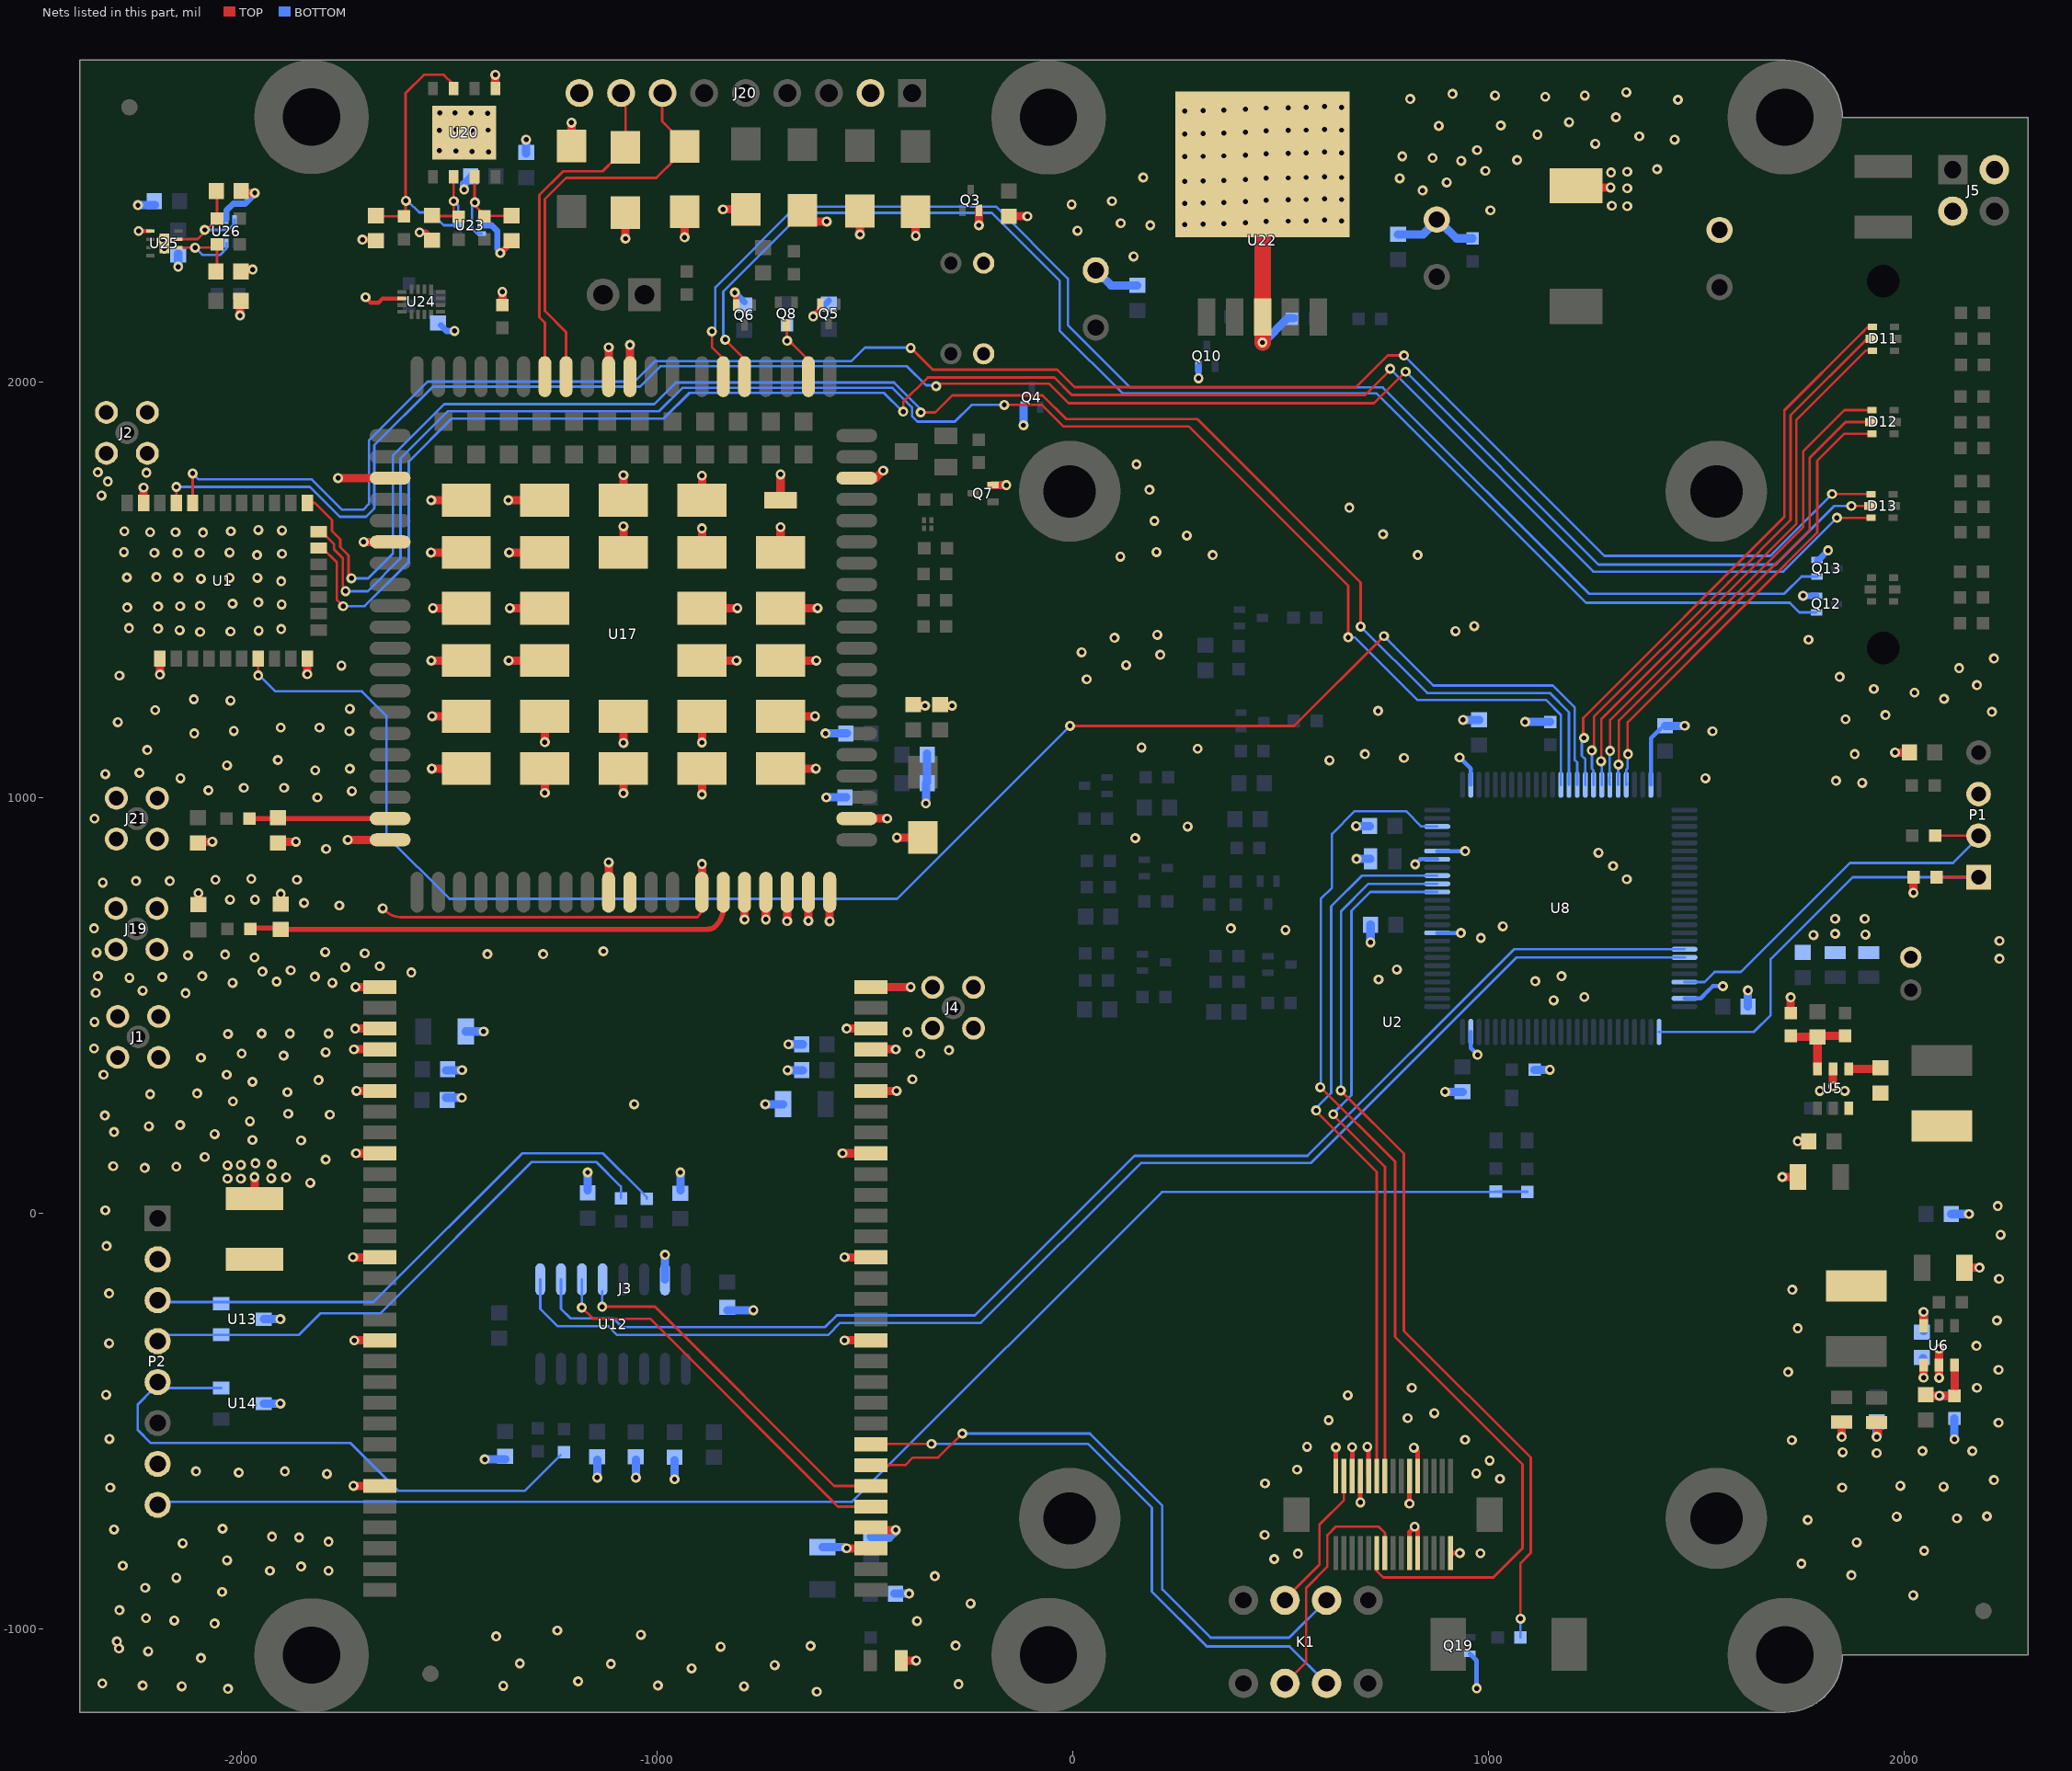
[diagram p0: the nets of this part, all layers, seen from the top]
# Altium PCB MISC84456.PcbDoc (part 3 of 5)
Units mil, origin at the board's own origin, x right, y up, seen from the top; angles counter-clockwise.
Board outline 4685.04 x 3973.82 mil, 4 copper layers (TOP, GND, POWER, BOTTOM), stack 38.4 mil thick; 219 components, 175 nets, 938 pads, 792 vias.

## Via types
v1: diameter 24, hole 12, TOP to BOTTOM, 400 vias
v2: diameter 24, hole 12, TOP to BOTTOM, tented both sides, 388 vias
v3: diameter 40, hole 20, TOP to BOTTOM, 4 vias

## Nets (pads, with @x,y where several pads share a name; then routed paths per layer and width w, separated by ;. In a path a pad name is that pad's centre, name@x,y a point inside that pad or via, vN(x,y) a via of type N, cw(c..) or ccw(c..) an arc to the next point about the centre after c; other vN are vias at no path point) (continued)
232RX-GPS: P2.4 R60.1 U13.1 | length 1332.6
  BOTTOM w6: P2.4@-2194,-293 -2193,-292 -1862,-292 -1810,-240 -1666,-240 -1302,124 -1146,124 -1087,65 R60.1@-1087,36.6
232TX-DB: P2.5 R61.1 U14.2 | length 1381
  BOTTOM w6: P2.5@-2213,-423 -2249,-459 -2249,-520 -2217,-552 -1737,-552 -1622,-667 -1318,-667 R61.1@-1232,-581 ; P2.5@-2201,-413 -2194.4,-419.6 U14.2@-2048.18,-419.6
232TX-GPS: P2.3 R59.1 U13.2 | length 1356.4
  BOTTOM w6: P2.3@-2184,-216 -2181,-213 -1682,-213 -1324,145 -1130,145 -1025,40 R59.1@-1025,35.6
433_CH_SW: R57.2 U8.16 | length 2204.2
  TOP w6: v1(644,296) v1@650.5,289.5 ; v1@647.5,292.5 v1@650.5,289.5 ; v1(1076.5,-974.5) 1076.5,-840.5 1101,-816 1101,-587 796,-282 796,144 v1@650.5,289.5
  BOTTOM w6: v1@645,300 645,727 711.18,793.18 U8.16@876.11,793.18 ; R57.2@1076.5,-1019 v1(1076.5,-974.5)
433_M0: U2.11 U8.17 | length 1875.7
  TOP w6: v1@576,247 578,245 586,245 730.63,100.37 730.63,-129 ; U2.11@730.63,-631.48 730.63,-129 ; 730.63,1.37 730.63,-129
  BOTTOM w6: v1(585,248) 579,248 621,290 ; 621,292 621,739 694.86,812.86 U8.17@876.11,812.86
433_RTK_RX: J3.37 K1.2 | length 1504.3
  TOP w6: J3.37@-485.45,-605 -436,-605 ; -417,-605 -436,-605 ; v1(-266,-529) -324,-587 -385,-587 -403,-605 -436,-605
  BOTTOM w6: v1(-266,-529) 41,-529 215,-703 215,-904 331,-1020 520,-1020 K1.2@610,-930
433_RTK_TX: J3.38 K1.7 | length 1459.9
  TOP w6: J3.38@-455,-554 -430,-554 ; -392,-554 -430,-554 ; v1(-340,-554) -430,-554
  BOTTOM w6: v1(-340,-554) 37,-554 190,-707 190,-909 322,-1041 521,-1041 K1.7@610,-1130
433_RX: K1.3 U2.3 | length 345.8
  TOP w6: K1.3@516,-921 593,-844 593,-748 651.89,-689.11 U2.3@651.89,-631.48
433_SIGNAL: U2.12 U8.23 | length 2654
  TOP w6: v1@594,306 775,125 775,-297 1081,-603 1081,-805 1011,-875 746,-875 730.63,-859.63 U2.12@730.63,-816.52
  BOTTOM w6: v1(595,304) 596,304 596,757 623,784 623,913 678,968 801,968 838.03,930.97 U8.23@876.11,930.97
433_SW: U2.13 U8.15 | length 1657.9
  TOP w6: v1@622.5,240.5 750.31,112.69 U2.13@750.31,-631.48
  BOTTOM w6: v1@624,239 670,285 670,728 715.49,773.49 U8.15@876.11,773.49
  other v1: 626,239
433_TX: K1.6 U2.14 | length 591.9
  TOP w6: K1.6@516,-1124 561,-1079 561,-900 612,-849 612,-773 632,-753 735,-753 750.31,-768.31 U2.14@750.31,-816.52
ACIN: J5.3
ANT_DIV: C103.2 R64.1 U17.35 | length 376.5
  TOP w12.5: R64.1@-1980.5,950 -1944,950 ; -1937,950 -1944,950 ; C103.2@-1903,950 C103.2@-1895,950 ; U17.35@-1679,950.09 U17.35@-1642.02,950.09 ; U17.35@-1656,950 -1944,950
ANT_GNSS: U17.47
ANT_MAIN: C98.2 R62.1 U17.49 | length 1175.6
  TOP w12.5: R62.1@-1978.5,685 -1978.5,687 C98.2@-1901,687 ; C98.2@-1905,683.69 -876.31,683.69 ; -877,684 ccw(c-877,707.9) -860.1,691 ; -859,692 ccw(c-902.84,735.84) U17.49@-840.84,735.84
AP_READY_MODULE: Q8.3 R30.2 U17.2 | length 171.9
  TOP w6: v2(-687.3,2099.3) Q8.3@-687.3,2129.3 ; v2@-682,2099 -664.5,2081.5 -636.12,2053.12 U17.2@-636.12,2013.08
  BOTTOM w6: v2(-687.3,2099.3) R30.2@-687.3,2136.3
BLE_RST: U1.7 U8.40 | length 4123.3
  TOP w6: v1(-1959.35,1294.35) U1.7@-1959.35,1334.99 ; v1(-7,1173) 532,1173 v1(748,1389)
  BOTTOM w6: v1(-1959.35,1294.35) v1@-1954,1294.35 ; v1@-1954,1292 -1918,1256 -1710,1256 -1651,1197 -1651,909 -1499,757 -423,757 v1(-7,1173) ; v1(748,1389) 773.5,1363.5 ; 770,1367 773.5,1363.5 ; U8.40@1212.72,1031.36 1212.72,1085.28 1207,1091 1207,1217 1154,1270 867,1270 773.5,1363.5
BLE_SLP: U1.17 U8.38 | length 4041.4
  TOP w6: U1.17@-1813.69,1640.11 -1806.86,1640.11 -1777,1610.25 -1777,1598 -1756,1577 v1@-1756,1504 ; v1@-165,1944 v1@-163,1946 ; v1@-162,1945 -74,1945 -22,1893 279,1893 662,1510 v1(662,1386)
  BOTTOM w6: v1(-1749,1497) -1696,1497 -1617,1576 -1617,1816 -1503,1930 -995,1930 -939,1986 -434,1986 -387,1939 -387,1918.3 -373.7,1905 -284,1905 -244,1945 v1(-165,1945) ; v1(662,1386) 678,1386 829,1235 1138.23,1235 1173.35,1199.87 U8.38@1173.35,1031.36
BLE_SW: U1.18 U8.39 | length 4087
  TOP w6: U1.18@-1841.24,1709.01 -1823.01,1709.01 -1782,1668 -1782,1642 -1762,1622 -1762,1603 -1742,1583 v1@-1742,1535 ; v1@-362,1927 -331,1927 -290,1968 -73,1968 -16,1911 299,1911 692,1518 v1(692,1412)
  BOTTOM w6: v1(-1735,1528) -1695,1528 -1635,1588 -1635,1824 -1512,1947 -1007,1947 -955,1999 -430,1999 -366,1935 v1(-366,1927) ; v1(692,1412) 852,1252 1147,1252 1193.04,1205.96 U8.39@1193.04,1031.36
BOOT0: P2.8 R37.2 R38.1 | length 3595.1
  BOTTOM w6: P2.8@-2196,-694 -2195,-693 -531,-693 214,52 1015.5,52 R38.1@1017,53.5 ; R38.1@1020.5,52.5 R37.2@1093,52.5
CPU-URX0: U8.69 U12.9 | length 3286.8
  BOTTOM w6: -1281,-219 U12.9@-1281,-158.2 -1281,-229 -1239,-271 -1117,-271 -1096,-292 -589,-292 -560,-263 -221,-263 164,122 573,122 1067,616 U8.69@1472,616
CPU-UTX0: U8.68 U12.10 | length 3167
  BOTTOM w6: U12.10@-1231,-158.2 -1231,-229 -1208,-252 -1105,-252 -1084,-273 -596,-273 -568,-245 -236,-245 148,139 564,139 1060.69,635.69 U8.68@1470.59,635.69
DBG_RXD: D18.2 J20.7 U17.11 | length 898.7
  TOP w6: U17.11@-1219,2038 -1219,2120 -1269.98,2170.98 -1269.98,2440.02 -1219,2491 -1001,2491 -1001,2492 D18.2@-955,2538 ; J20.7@-988,2670 -988,2627 D18.2@-934,2573
DBG_TXD: D19.2 J20.8 U17.12 | length 773.6
  TOP w6: U17.12@-1269.98,2013.08 -1269.98,2142.98 -1283,2156 -1283,2450 -1226,2507 -1131,2507 D19.2@-1101,2537 ; D19.2@-1076,2564.74 J20.8@-1076,2678
DBG_TXD_FC20: J20.9
GND: C1.1 C2.2 C3.2 C4.2 C5.1 C6.2 C7.2 C8.1 C9.1 C10.1 C11.2 C20.1 C21.1 C22.1 C24.2 C26.2 C27.2 C28.2 C29.2 C30.1 C31.1 C32.2 C34.2 C35.2 C36.2 C37.2 C38.1 C40.2 C41.2 C42.2 C43.2 C44.1 C45.2 C46.1 C47.2 C48.2 C49.2 C50.2 C51.2 C52.2 C53.2 C54.2 C55.1 C56.2 C70.2 C71.2 C72.2 C73.2 C74.2 C75.2 C76.2 C77.2 C88.2 C91.2 C92.2 C94.1 C95.1 C96.2 C97.1 C98.1 C99.2 C100.2 C101.2 C102.1 C103.1 C104.2 C105.2 D3.1 D7.2 D8.1 D14.1 D15.1 D16.1 D17.1 D18.1 D19.1 D24.1 J1.2 J1.3 J1.4 J1.5 J2.2 J2.3 J2.4 J2.5 J3.1 J3.3 J3.4 J3.6 J3.9 J3.14 J3.18 J3.25 J3.33 J3.34 J3.43 J3.47 J3.52 J3.55 J3.57 J3.58 J3.60 J4.2 J4.3 J4.4 J4.5 J5.2 J19.2 J19.3 J19.4 J19.5 J20.2 J21.2 J21.3 J21.4 J21.5 L2.2 P1.3 P2.7 Q3.2 Q4.2 Q5.2 Q6.2 Q7.2 Q10.2 Q12.2 Q13.2 Q19.1 R4.1 R7.2 R13.1 R20.1 R36.1 R42.1 R67.1 R68.1 U1.1 U1.10 U1.28 U2.1 U2.5 U2.7 U2.9 U2.19 U2.20 U2.21 U2.22 U2.30 U5.2 U6.2 U8.10 U8.19 U8.20 U8.27 U8.49 U8.74 U8.99 U12.15 U13.3 U14.3 U17.8 U17.9 U17.19 U17.22 U17.36 U17.46 U17.48 U17.50 U17.51 U17.52 U17.53 U17.54 U17.56 U17.72 U17.85 U17.86 U17.87 U17.88 U17.89 U17.90 U17.91 U17.92 U17.93 U17.94 U17.95 U17.96 U17.97 U17.98 U17.99 U17.100 U17.101 U17.102 U17.103 U17.104 U17.105 U17.106 U17.107 U17.108 U17.109 U17.110 U17.111 U17.112 U20.1 U20.9 U22.3 U22.6 U23.2 U24.6 U25.1 U25.9 U26.2 | length 11053.5
  TOP w6: v1@-1654,729 ccw(c-1615.37,767.63) -1615.37,713 -903,713 ccw(c-929.5,739.5) -892.02,739.5 U17.48@-892.02,772.92
  TOP w10: v2(-2246.92,2363.08) U25.1@-2218.15,2363.08 ; v2(-1701,2204) -1688,2191 -1670,2191 -1660.13,2200.87 U24.6@-1613.41,2200.87
  TOP w11: U2.5@671.57,-631.48 v1(671.57,-561.57) ; v1(691.26,-694.74) U2.7@691.26,-631.48 ; v1(708,-561) 710.94,-563.94 U2.9@710.94,-631.48 ; U2.20@809.37,-816.52 809.37,-765.63 v1@817,-758 ; v1(809.37,-697.63) U2.19@809.37,-631.48 ; v1(820,-563) 829.06,-572.06 U2.21@829.06,-631.48 ; v1(822,-753) 829.06,-760.06 U2.22@829.06,-816.52 ; U2.30@907.8,-816.52 v1(930.52,-816.52)
  TOP w12: U2.1@632.2,-631.48 v1(632.2,-562.2)
  TOP w15: v2(-1708.5,2342.5) C37.2@-1676,2342.5 ; v2(-1571,2360) -1557.5,2360 C36.2@-1541,2343.5 ; v2(-1377,2310) -1356,2331 C35.2@-1356,2343.5 ; v2(-813,2215.5) -810.12,2212.62 Q6.2@-810.12,2184.87 ; v2(-624.5,2158) -608,2174.5 Q5.2@-608,2181
  TOP w20: U1.28@-2234.94,1709.01 v1(-2234.94,1746.06) ; v1(-2195.57,1296.43) U1.1@-2195.57,1334.99 ; C102.1@-2104,894.5 v2(-2069.5,894.5) ; C97.1@-2103,740.5 v2(-2103,771) ; C51.2@-2003.18,2270.56 v2(-1972.44,2270.56) ; C50.2@-2003.18,2454.56 v2(-1967.56,2454.56) ; v2(-2003,2160) C52.2@-2003,2201 ; L2.2@-1968,36.97 v2(-1968,88) ; C103.1@-1912,894.5 v2(-1868.5,894.5) ; C98.1@-1905,741.5 v2(-1905,769) ; v1(-1841.24,1297.24) U1.10@-1841.24,1334.99 ; v2(-1767.02,1768.98) U17.19@-1642.02,1768.98 ; v2(-1744.09,898.91) U17.36@-1642.02,898.91 ; v2(-1731,-105) J3.14@-1666.55,-105 ; v1(-1730,-655) J3.25@-1666.55,-655 ; v2(-1729,395) J3.4@-1666.55,395 ; v2(-1728,-305) J3.18@-1666.55,-305 ; v2(-1726,445) J3.3@-1666.55,445 ; v2(-1725,545) J3.1@-1666.55,545 ; v2(-1724,145) J3.9@-1666.55,145 ; v2(-1723,295) J3.6@-1666.55,295 ; v2(-1705.56,1615.44) U17.22@-1631.02,1615.44 ; v2(-1543.85,1589.85) U17.107@-1458.95,1589.85 ; v2(-1543.17,1715.83) U17.112@-1458.95,1715.83 ; v2(-1542.99,1330.01) U17.98@-1458.95,1330.01 ; v2(-1541.83,1070.17) U17.89@-1458.95,1070.17 ; v2(-1540.85,1196.15) U17.94@-1458.95,1196.15 ; v2(-1538.99,1455.99) U17.102@-1458.95,1455.99 ; U20.1@-1389,2706.3 v2(-1389,2739) ; R42.1@-1372,2185.5 v2(-1372,2217) ; v2(-1357.83,1715.83) U17.111@-1269.98,1715.83 ; v2(-1357.01,1330.01) U17.97@-1269.98,1330.01 ; v2(-1355.85,1589.85) U17.106@-1269.98,1589.85 ; v2(-1353.99,1455.99) U17.101@-1269.98,1455.99 ; v2(-1269.98,1012.02) U17.88@-1269.98,1070.17 ; v2(-1269.98,1133.98) U17.93@-1269.98,1196.15 ; D24.1@-1206,2567.74 v2(-1206,2624) ; U17.46@-1116.43,772.92 v2(-1116.43,844.57) ; U17.9@-1116.43,2013.08 v2@-1116.43,2081.43 ; v2(-1081,1011) U17.87@-1081,1070.17 ; v2(-1081,1132) U17.92@-1081,1196.15 ; U17.105@-1081,1589.85 v2(-1081,1653) ; U17.110@-1081,1715.83 v2(-1081,1776) ; v2(-1076,2345) D19.1@-1076,2407.26 ; U17.8@-1065.25,2013.08 v2(-1065.25,2089.25) ; v2(-934,2348) D18.1@-934,2409.26 ; U17.48@-892.02,772.92 v2(-892.02,840.98) ; v2(-892.02,1008.02) U17.86@-892.02,1070.17 ; v2(-892.02,1132.98) U17.91@-892.02,1196.15 ; U17.96@-892.02,1330.01 v2(-809.01,1330.01) ; U17.100@-892.02,1455.99 v2(-807.01,1455.99) ; U17.104@-892.02,1589.85 v2(-892.02,1647.98) ; U17.109@-892.02,1715.83 v2(-892.02,1774.98) ; v2(-841.74,2415.26) D14.1@-787,2415.26 ; v2(-789.66,707.34) U17.50@-789.66,772.92 ; v2(-738.48,707.48) U17.51@-738.48,772.92 ; U17.85@-703.05,1070.17 v2(-618.17,1070.17) ; U17.90@-703.05,1196.15 v2(-620.15,1196.15) ; U17.95@-703.05,1330.01 v2(-617.01,1330.01) ; U17.99@-703.05,1455.99 v2(-614.01,1455.99) ; U17.103@-703.05,1589.85 v2(-703.05,1651.05) ; U17.108@-703.05,1715.83 v2(-703.05,1777.95) ; v2(-687.3,703.3) U17.52@-687.3,772.92 ; D15.1@-651,2413.26 -651,2396 -641,2386 v2(-592,2386) ; v2(-636.12,704.12) U17.53@-636.12,772.92 ; v2(-584.94,703.06) U17.54@-584.94,772.92 ; v2(-554,145) J3.52@-485.45,145 ; v2(-549,-305) J3.43@-485.45,-305 ; v2(-549,-105) J3.47@-485.45,-105 ; v2(-544,-805) J3.33@-485.45,-805 ; v2(-544,445) J3.58@-485.45,445 ; U17.56@-519.98,950.09 v2(-446.91,950.09) ; U17.72@-519.98,1768.98 -474.02,1768.98 v2(-456,1787) ; v2(-512,2355) D16.1@-512,2411.26 ; J3.34@-485.45,-755 -479.45,-761 v2(-426,-761) ; J3.55@-485.45,295 v2(-424,295) ; J3.57@-485.45,395 v2(-426,395) ; J3.60@-485.45,545 v2(-390,545) ; v2(-423.26,904.26) D8.1@-361,904.26 ; D7.2@-412.6,-1075 v2(-377,-1075) ; C73.2@-384,1221.5 v2(-355.5,1221.5) ; v2(-378,2352) D17.1@-378,2409.26 ; C74.2@-319,1221.5 v2(-290.5,1221.5) ; v1(-226,2377) Q3.2@-226,2413.38 ; Q7.2@-192.38,1752 v1(-160,1752) ; C32.2@-154,2398.69 v1(-109.68,2398.69) ; D3.1@1231.13,2468 v2(1293,2468) ; v2(1706,88) C30.1@1743.84,88 ; R13.1@1726,482.5 v2(1726,520) ; v2(1743,174) C31.1@1772.5,174 ; v2(1828,306) U5.2@1828,347.89 ; v2(1849,-537) C42.2@1849,-501.53 ; v2(1933,-537) 1936,-534 C40.2@1936,-508 ; v1(1977,1109) C1.1@2011.69,1109 ; v1(2021.5,771.5) R7.2@2021.5,809 ; v2(2083,-395) U6.2@2083,-364.24 v2(2083,-325) ; C44.1@2144.16,-130 v2(2180,-130)
  TOP w40: v2(456,2095) U22.3@456,2156.23 U22.6@456,2349
  BOTTOM w10: v2(-1701,2204) v2@-1701,2205 ; v1(823,840) 835.23,852.23 U8.19@876.11,852.23 ; U8.10@876.11,675.06 v1(932.94,675.06) ; U8.20@876.11,871.92 v1(943.08,871.92) ; v1(930,1097) 929,1098 956.81,1070.19 U8.27@956.81,1031.36 ; U8.99@956.81,436.88 956.81,398.19 v1(973,382) ; U8.49@1389.89,1031.36 1389.89,1143.89 C3.2@1412,1166 ; U8.74@1470.59,517.58 1509.58,517.58 1527,535 1539,547 v1(1563,547)
  BOTTOM w11: Q19.1@954.56,-1058.68 971,-1075.13 v1(971,-1142)
  BOTTOM w15: U26.2@-2035.68,2391 -2035.68,2412.32 -2019,2429 -1991,2429 v2@-1970,2450 ; C38.1@-1519.5,2136.5 -1506,2123 v2(-1487,2123) ; U23.2@-1421.56,2377 -1398,2377 -1384,2363 -1384,2320 v2@-1377,2313 ; v2(-813,2215.5) C48.2@-790,2192.5 ; v2(-624.5,2158) C47.2@-587,2195.5 ; v1(302,2009) Q10.2@302,2038.38 ; v1(1756,1486) Q12.2@1788.38,1486 ; Q13.2@1789.38,1572 1793,1572 v1(1816,1595)
  BOTTOM w20: v2(-2248.44,2425.56) C45.2@-2207.18,2425.56 ; v2(-2151.68,2277.32) C49.2@-2151.68,2308.06 ; U14.3@-1945.82,-457 v1(-1906,-457) ; U13.3@-1945.82,-254 v1(-1906,-254) ; C8.1@-1507.62,278.76 v2(-1469.75,278.76) ; C9.1@-1507.5,345 v2(-1469,345) ; v2(-1464,2463) -1464,2476.5 C34.2@-1445.5,2495 ; C10.1@-1459.84,438 v2(-1417,438) ; v2(-1414.3,-591.3) C99.2@-1365,-591.3 ; C24.2@-1315,2549.5 v2(-1315,2583) ; C95.1@-1167,56.5 v2(-1167,99) ; v2(-1144,-635) C100.2@-1144,-592.3 ; v2(-1051,-635) C96.2@-1051,-592.4 ; U12.15@-981,-158.2 v2(-981,-99) ; v2(-958,-639) C92.2@-958,-593.4 ; C94.1@-944,55.5 v2(-944,99) ; C88.2@-831,-232.4 v2(-768.4,-232.4) ; v2(-740,263) C5.1@-697.16,263 ; v2(-686.24,344.76) C6.2@-649.62,344.76 ; v2(-684,407) C7.2@-649.5,407 ; C22.1@-602,-801.84 -551.16,-801.84 v2@-548,-805 ; v2(-595,1155) C72.2@-543.5,1155 ; v2(-593,1001) C75.2@-545.5,1001 ; C20.1@-486,-777 -483,-780 -442,-780 v2@-426,-764 ; C21.1@-429.5,-914 v2(-394,-914) ; v2(-353.5,986.5) -353.5,1035 -351,1037.5 C71.2@-351,1106 ; v1(-119,1896) Q4.2@-119,1939.38 ; C91.2@67,2257 91.69,2232.32 C101.2@155,2232.32 ; v2@458.5,2097.5 v2(456,2095) 458,2095 517,2154 R68.1@531,2154 ; v2@459,2096 v2@460,2096 ; v1(681,932) C56.2@713.69,932 ; v1(682,853) C55.1@715.47,853 ; v1(715.69,652.32) C54.2@715.69,695 ; C105.2@782,2355.32 842.32,2355.32 C104.2@868,2381 ; C104.2@891,2377 922.5,2345.5 R67.1@961,2345.5 ; v1(895.32,292.69) C11.2@937,292.69 ; v1(938.32,1187.32) C2.2@977,1187.32 ; v1(1087.5,1182.5) R4.1@1148,1182.5 ; R36.1@1110.5,346 v1(1147,346) ; C3.2@1424,1173.32 v1(1471.32,1173.32) ; C53.2@1623.32,498 v1(1623.32,536.69) ; v2@1849,-532 C43.2@1849,-501.53 ; v2(1933,-537) C41.2@1933,-498.5 ; v2@2086,-325 v2@2086.5,-325.5 ; C46.1@2112.32,-1 v1(2155,-1) ; v2(2120,-543) R20.1@2120,-492.5
  other v1: -2097,-1069 -2224,-1053 -2294,-1046 -2299,-1029 -2064,-986 -2161,-979 -2229,-973 -2293,-954 2021,-918 -2046,-910 -2231,-900 -2156,-876 1872,-870 -1931,-859 -1790,-859 -1856,-849 -2285,-847 1752,-842 -2034,-834 484,-831 541,-818 980,-817 2047,-811 1885,-791 -1790,-789 -1861,-779 -1926,-777 461,-773 1767,-737 2126,-733 1981,-729 2198,-728 1850,-659 2094,-657 1990,-655 462,-649 2215,-641 1027,-638 -1794,-626 970,-625 -2006,-623 -2109,-620 -1895,-620 539,-616 1002,-594 563,-561 1729,-545 943,-544 2226,-503 615,-497 805,-492 869,-480 661,-437 815,-419 1720,-381 2226,-376 1743,-276 2222,-257 1730,-183 2227,-157 2231,-51 2224,18 -1834,74 -1797,130 -2088,136 -1856,176 -1973,177 -2064,191 -2222,210 -2147,213 -1979,222 -1787,238 -1887,240 -2020,270 -2219,287 -1814,321 -2035,334 -2032,432 -1951,433 -1883,433 -1790,433 1156,513 1230,521 -2134,530 -2237,536 -1781,555 -1915,558 1112,559 735,563 1175,571 779,587 -1750,592 -1408,624 -1274,624 -1703,626 -1129,631 981,663 1781,670 1906,671 511,682 380,686 1034,691 1833,709 -1660,734 -1764,741 -2027,755 -1967,755 1332,804 1299,836 1264,868 150,903 276,931 1898,1036 1835,1041 1521,1047 -1822,1066 -2034,1078 617,1090 -1912,1091 796,1096 702,1105 1880,1105 -2226,1115 300,1118 165,1121 -2113,1155 1538,1160 -2018,1161 -1905,1169 -1812,1169 -2297,1182 1858,1189 1954,1199 2210,1207 734,1209 -2207,1211 -2026,1234 -2114,1237 2095,1238 2024,1253 1926,1262 2174,1271 33,1285 1844,1291 -2293,1294 2131,1312 128,1319 2215,1335 210,1344 21,1350 1769,1380 100,1385 203,1392 -2099,1399 -2026,1400 920,1401 -1958,1402 -2148,1403 -1904,1406 -2200,1407 -2270,1408 965,1413 -2274,1458 -2200,1460 -2147,1461 -2099,1462 -1903,1465 -2021,1467 -1959,1470 -1904,1521 -2097,1527 -2028,1529 -1961,1529 -2275,1530 -2151,1530 -2204,1531 114,1580 -1962,1584 336,1584 829,1584 -1902,1587 -2209,1589 -2153,1589 -2100,1589 -2028,1590 -2282,1591 201,1591 274,1631 746,1634 -2092,1638 -2219,1639 -2158,1639 -2281,1641 -2025,1641 -1902,1643 -1959,1644 196,1666 665,1698 -2336,1727 184,1741 -2321,1761 -2228,1782 -2345,1783 153,1802 146,2302 11,2364 186,2377 115,2382 1004,2413 -3,2427 94,2435 841,2461 899,2480 786,2490 169,2492 992,2508 1405,2512 934,2532 1068,2534 865,2539 792,2543 972,2558 1256,2573 1447,2583 1362,2591 1117,2595 880,2616 1029,2617 1193,2625 1306,2637 1455,2679 811,2681 1136,2686 1015,2689 1231,2689 913,2693 1331,2697
  other v2: -616,-1150 -2032,-1143 -2143,-1137 -791,-1137 -1370,-1136 -2237,-1135 -998,-1135 -275,-1132 -2334,-1130 -1190,-1125 -917,-1094 -717,-1086 -1111,-1083 -1330,-1082 -847,-1042 -631,-1040 -282,-1039 -1387,-1017 -1039,-1013 -1240,-1003 -375,-980 -246,-938 -332,-872 -2141,-793 -2306,-760 -2045,-758 -2315,-659 1933,-576 1851,-574 2043,-571 2163,-571 -2317,-542 -2325,-436 2174,-419 2173,-318 -2318,-312 -2318,-192 -2324,-78 -2327,8 -2033,84 -2001,84 -1928,85 -1892,87 -2232,110 -2156,113 -2308,114 -2033,116 -2001,117 -1927,119 -1966,121 -2306,196 -2328,236 -1055,263 -2106,289 -1889,292 1796,295 1856,295 -1973,317 -386,323 -2331,334 -2097,375 -1898,380 -1999,385 -367,385 -1797,388 -298,393 -2354,397 -398,436 -2353,461 -2350,531 -2021,555 -2269,567 -2190,569 -1823,570 -2345,571 -2094,571 -1591,580 -1949,582 -1881,585 -1667,595 2228,613 -1968,616 -2128,621 -2039,623 -2348,628 -1798,629 2228,656 1833,673 -2354,686 1904,709 -1849,747 -2333,796 -2253,800 -2172,800 -2062,803 -1866,803 -1976,805 -1796,877 -2353,950 -1817,1001 -1734,1016 -2079,1018 -1994,1024 -1897,1024 -2146,1047 -2327,1057 -2245,1060 -1739,1070 -1740,1160 -1739,1214 -1759,1318 -1116.43,2083.57 -2185,2321 -2189,2343 269,2379 313,2380 363,2381 415,2383 465,2386 518,2387 561,2388 646,2388 605,2390 1333,2423 1296,2424 269,2430 313,2431 363,2432 415,2434 465,2437 518,2438 561,2439 646,2439 605,2441 1333,2466 269,2483 313,2484 363,2485 415,2487 465,2490 518,2491 561,2492 646,2492 605,2494 1294,2504 1333,2506 269,2542 313,2543 363,2544 415,2546 465,2549 518,2550 561,2551 646,2551 -1405,2553 605,2553 -1445,2555 -1484,2556 -1524,2557 269,2597 313,2598 363,2599 415,2601 465,2604 -1524,2605 -1446,2605 518,2605 -1406,2606 561,2606 646,2606 -1484,2607 605,2608 -1407,2646 -1522,2647 -1486,2647 -1447,2647 269,2652 313,2653 363,2654 415,2656 465,2659 518,2660 561,2661 646,2661 605,2663
GND_IN: L2.1 P2.2
GPS_RXD1: J3.36 U12.12 | length 862.1
  TOP w6: v2(-1132,-224) -1005,-224 -574,-655 J3.36@-485.45,-655
  BOTTOM w6: v2(-1132,-224) U12.12@-1132,-187
GPS_TXD1: J3.35 U12.11 | length 961.8
  TOP w6: v2(-1181,-226) -1154,-253 -1017,-253 -579,-691 -577,-693 -565,-705 J3.35@-485.45,-705
  BOTTOM w6: v2(-1181,-226) U12.11@-1181,-158.2
JTCK: P1.1 R7.1 U8.76 | length 1086.1
  TOP w6: R7.1@2076.5,809 P1.1@2164,809
  BOTTOM w6: U8.76@1409.57,436.88 1637.88,436.88 1678,477 1678,612 1875,809 P1.1@2175,809
JTMS: P1.2 R25.1 U8.72 | length 943.4
  TOP w6: R25.1@2073.5,909 P1.2@2171,909
  BOTTOM w6: U8.72@1470.59,556.95 1518.95,556.95 1543,581 1606,581 1868.5,843.5 2116.5,843.5 P1.2@2174,901
LED1_B: D11.5 U8.41 | length 1398.2
  TOP w6: v1@1227,1147 1227,1192 1711,1676 1711,1932 1896.57,2117.57 1896.69,2117.57 1911.67,2132.54 D11.5@1922.42,2132.54
  BOTTOM w6: v1(1229,1144) 1224,1139 1224,1101 1232.41,1092.59 U8.41@1232.41,1031.36
LED1_G: D11.1 U8.43 | length 1332.3
  TOP w6: v1@1272,1081 1271,1082 1271,1190 1740,1659 1740,1909 1906.46,2075.46 D11.1@1922.42,2075.46
  BOTTOM w6: v1(1270,1088) 1270,1083 1269,1082 1271.78,1079.22 U8.43@1271.78,1031.36
LED1_R: D11.3 U8.42 | length 1361
  TOP w6: v1@1247,1115 1253,1121 1253,1195 1578.5,1520.5 ; 1576,1518 1578.5,1520.5 ; D11.3@1919.47,2104 1910,2104 1726,1920 1726,1668 1578.5,1520.5
  BOTTOM w6: v1(1248,1114) 1248,1070 1252.09,1065.91 U8.42@1252.09,1031.36
LED2_B: D12.5 U8.44 | length 1210.5
  TOP w6: v1@1292,1106 v1(1292,1113) 1292,1187 1756,1651 1756,1833 1855.54,1932.54 D12.5@1921.42,1932.54
  BOTTOM w6: U8.44@1290.15,1049 1290.15,1032.67 U8.44@1291.46,1031.36 ; v1@1290.15,1111.15 v1(1292,1113) ; U8.44@1292,1049 1291,1050 1291,1111 v1@1292,1112
LED2_G: D12.1 U8.46 | length 1129.3
  TOP w6: v1@1334,1109 1334,1182 1639,1487 ; 1636,1484 1639,1487 ; D12.1@1921.42,1875.46 1854.46,1875.46 1790,1811 1790,1638 1639,1487
  BOTTOM w6: v1@1330.83,1100.83 v1@1333,1098.67 ; U8.46@1333,1033.53 U8.46@1330.83,1031.36 1330.83,1067.83 1334,1071 v1@1334,1100
  other v1: 1335,1105
LED2_R: D12.3 U8.45 | length 1169.3
  TOP w6: v1@1311,1074 1313,1076 1313,1113 1313,1186 1618,1491 ; 1616,1489 1618,1491 ; D12.3@1918.47,1904 1858,1904 1772,1818 1772,1645 1618,1491
  BOTTOM w6: U8.45@1311.15,1031.36 1311.15,1079.85 1311.31,1080 v1(1312,1080)
LED3_B: D13.5 U1.25 | length 4721.3
  TOP w6: U1.25@-2116.83,1709.01 v1(-2116.83,1780.17) ; v1(-390,2082) -389,2082 -337,2030 -38,2030 4,1988 681,1988 757,2064 v1(796,2064) ; v1(1825.54,1730.54) D13.5@1919.42,1730.54
  BOTTOM w6: v1(-2116.83,1780.17) -2102.67,1766 -1830,1766 -1757,1693 -1715,1693 ; -1712,1693 -1715,1693 ; v1@-398,2083 -500,2083 -533,2050 -1005,2050 -1054,2001 -1552,2001 -1693,1860 -1693,1707 -1707,1693 -1715,1693 ; v1(796,2064) 1278,1582 1677,1582 v1(1825.54,1730.54)
LED3_G: D13.1 U1.16 | length 4571.6
  TOP w6: U1.16@-1813.69,1600.74 -1804.74,1600.74 -1770,1566 -1770,1476 v1(-1755,1461) ; v1(-408,1929) -408,1952 -349,2011 -45,2011 -3,1969 703,1969 763,2029 v1(763,2032) ; v1(1837.46,1673.46) D13.1@1919.42,1673.46
  BOTTOM w6: v1(-1755,1461) -1703,1461 -1597,1567 -1597,1809 -1494,1912 -984,1912 -922,1974 -469,1974 ; -459,1974 -469,1974 ; v1@-411,1930 -455,1974 -469,1974 ; v1(763,2032) 1251,1544 1708,1544 v1(1837.46,1673.46)
LED3_R: D13.3 U1.26 | length 4727.4
  TOP w6: U1.26@-2156.2,1709.01 v1(-2156.2,1747.8) ; v1@-329,1992 -325,1996 -57,1996 -10,1949 724,1949 v1(800,2025) ; v1(1872,1702) D13.3@1916.47,1702
  BOTTOM w6: v1(-2156.2,1747.8) -1834.8,1747.8 -1763,1676 -1719,1676 ; -1715,1676 -1719,1676 ; -475,2038 -497,2038 ; v1@-330,1992 -353,1992 -399,2038 -497,2038 ; v1(800,2025) 1264,1561 1690,1561 1831,1702 v1(1872,1702) ; -1719,1676 -1700,1676 -1680,1696 -1680,1848 -1539,1989 -1041,1989 -992,2038 -497,2038
  other v1: -329,1990
NET_MODE: Q12.1 U17.5 | length 3395.2
  TOP w6: v2(-836,2102) -789.66,2055.66 U17.5@-789.66,2013.08
  BOTTOM w6: v2@-840.84,2105 -840.84,2217.36 -651.2,2407 -195,2407 -32,2244 -32,2124 119,1973 730,1973 1234,1469 1724,1469 1747,1446 Q12.1@1787,1446
NET_STATUS: Q13.1 U17.6 | length 3427
  TOP w6: v2(-868,2122) -868,2084 -840.84,2056.84 U17.6@-840.84,2013.08
  BOTTOM w6: v2@-867,2122 -860,2129 -860,2228 -666,2422 -185,2422 -12,2249 -12,2137 138,1987 745,1987 1241,1491 1711,1491 1752,1532 Q13.1@1789.38,1532
NetC23_1: C23.1 L3.1 U5.6
NetC23_2: C23.2 U5.1 | length 71.7
  TOP w20: U5.1@1865.4,347.89 C23.2@1937.11,347.89
NetC25_2: C25.2 R11.1 R13.2 U5.3 | length 204.8
  TOP w20: R13.2@1731,425 1791,425 1790.6,424.6 U5.3@1790.6,347.89 ; C25.2@1791,427.5 R11.1@1858.5,427.5
NetC33_1: C33.1 L4.1 U6.6 | length 79.1
  TOP w20: U6.6@2045.6,-269.76 v2(2045.6,-236.4)
  BOTTOM w20: v2(2045.6,-236.4) 2046,-236.8 C33.1@2046,-282
NetC33_2: C33.2 U6.1 | length 77.6
  TOP w20: v2(2045.6,-394.6) U6.1@2045.6,-364.24
  BOTTOM w20: C33.2@2044,-348 2045.6,-349.6 v2(2045.6,-394.6)
NetC35_1: C35.1 R14.2 U20.7 U23.3 | length 251.7
  TOP w6: U20.7@-1439,2493.7 -1439,2426 -1413,2400 C35.1@-1360,2400
  BOTTOM w6: v2(-1438,2432) -1445,2425 -1445,2369 -1433.31,2357.32 U23.3@-1421.56,2357.32
NetC36_1: C36.1 R15.2 U20.6 U23.6 | length 180.8
  TOP w6: C36.1@-1533,2399 -1490,2399 -1489,2400 -1489,2433 U20.6@-1489,2493.7
  BOTTOM w6: v2(-1489,2435) -1478.44,2424.44 U23.6@-1478.44,2396.69
NetC37_1: C37.1 R16.2 U20.3 U23.5 | length 658.9
  TOP w6: C37.1@-1671.5,2398.5 R16.2@-1604,2398.5 ; R16.2@-1605,2401 -1605,2695 -1561,2739 -1513,2739 -1489,2715 U20.3@-1489,2706.3
  BOTTOM w6: v2@-1599,2435 -1572,2408 -1544,2408 -1513,2377 U23.5@-1478.44,2377
  other v2: -1604,2436
NetC39_2: C39.2 R17.1 R20.2 U6.3 | length 169.3
  TOP w20: C39.2@2060,-438 v2(2084,-438) 2086,-438 2119,-438 2120.4,-436.6 U6.3@2120.4,-364.24
  BOTTOM w20: v2(2084,-438) R20.2@2120,-438
NetC50_1: C50.1 R21.2 U25.7 U26.3 | length 255.7
  TOP w6: U25.7@-2151.22,2343.4 -2150.62,2344 -2105,2344 -2058,2391 C50.1@-2058,2446
  BOTTOM w6: v2(-2088,2366) -2031.72,2366 -2016,2381.72 U26.3@-2016,2391
NetC51_1: C51.1 R23.2 U25.6 U26.5 | length 242.3
  TOP w6: U25.6@-2151.22,2323.71 R23.2@-2069.71,2323.71 ; C51.1@-2058.18,2272.82 R23.2@-2058.18,2331.56
  BOTTOM w6: v2(-2111,2323) -2104,2316 -2094,2306 -2050,2306 -2035.68,2320.32 U26.5@-2035.68,2334.11